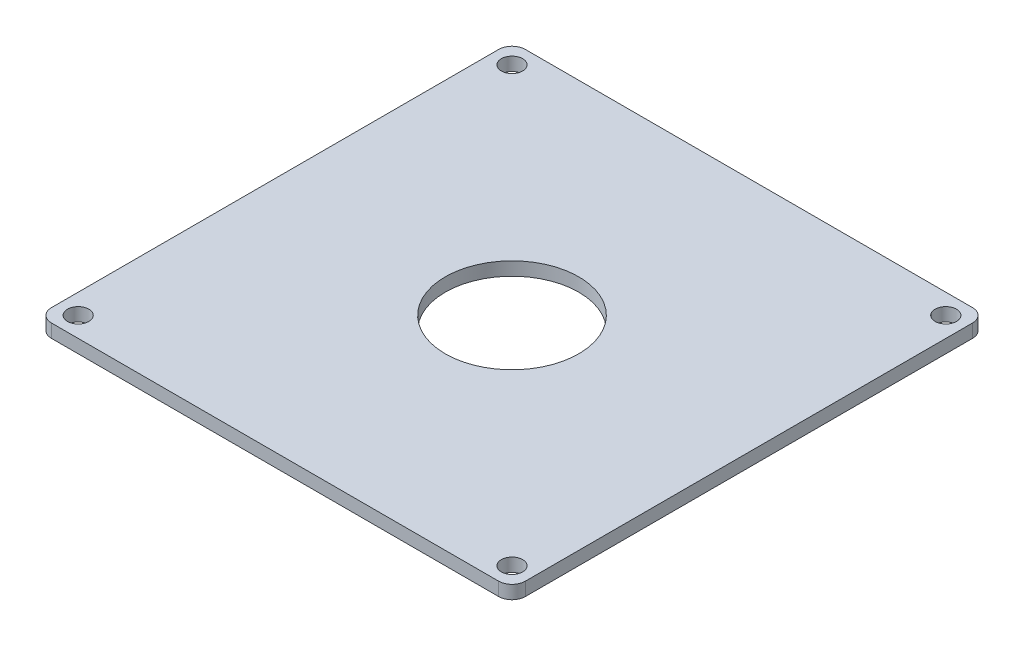
SolidWorks part; units mm, degrees
ref_plane "Front Plane" through (0, 0, 0) normal (0, 0, 1) x (1, 0, 0)
ref_plane "Top Plane" through (0, 0, 0) normal (0, 1, 0) x (1, 0, 0)
ref_plane "Right Plane" through (0, 0, 0) normal (1, 0, 0) x (0, 0, -1)
sketch "Sketch1" plane through (0, 0, 0) normal (0, 1, 0) x (1, 0, 0)
  line L1 (-32.5, -32.5) -> (32.5, -32.5) construction
  line L2 (-32.5, -32.5) -> (-32.5, 32.5) construction
  line L3 (-32.5, 32.5) -> (32.5, 32.5) construction
  line L4 (32.5, -32.5) -> (32.5, 32.5) construction
  line L5 (-32.5, -32.5) -> (32.5, 32.5) construction
  line L6 (-32.5, 32.5) -> (32.5, -32.5) construction
  line L7 (-33.5, -35.5) -> (33.5, -35.5)
  line L8 (-35.5, -33.5) -> (-35.5, 33.5)
  line L9 (-33.5, 35.5) -> (33.5, 35.5)
  line L10 (35.5, -33.5) -> (35.5, 33.5)
  line L11 (-35.5, -35.5) -> (35.5, 35.5) construction
  line L12 (-35.5, 35.5) -> (35.5, -35.5) construction
  circle A0 centre (-32.5, 32.5) radius 1.6
  circle A1 centre (32.5, 32.5) radius 1.6
  circle A2 centre (32.5, -32.5) radius 1.6
  circle A3 centre (-32.5, -32.5) radius 1.6
  arc A4 (-33.5, -35.5) -> (-35.5, -33.5) centre (-33.5, -33.5) cw
  arc A5 (33.5, -35.5) -> (35.5, -33.5) centre (33.5, -33.5) ccw
  arc A6 (33.5, 35.5) -> (35.5, 33.5) centre (33.5, 33.5) cw
  arc A7 (-35.5, 33.5) -> (-33.5, 35.5) centre (-33.5, 33.5) cw
  point P0 (0, 0)
  point P6 (0, 0)
  dimension "D3" = 3.2
  dimension "D4" = 3.2
  dimension "D5" = 3.2
  dimension "D6" = 3.2
  dimension "D9" = 2
  dimension "D1" = 65
  dimension "D2" = 65
  dimension "D7" = 71
  dimension "D8" = 71
extrude "Boss-Extrude1" add sketch "Sketch1" along normal blind 2
sketch "Sketch2" plane through (0, 2, 0) normal (0, 1, 0) x (1, 0, 0)
  circle A0 centre (0, 0) radius 10
  dimension "D1" = 20
extrude "Cut-Extrude1" cut sketch "Sketch2" against normal blind 10
